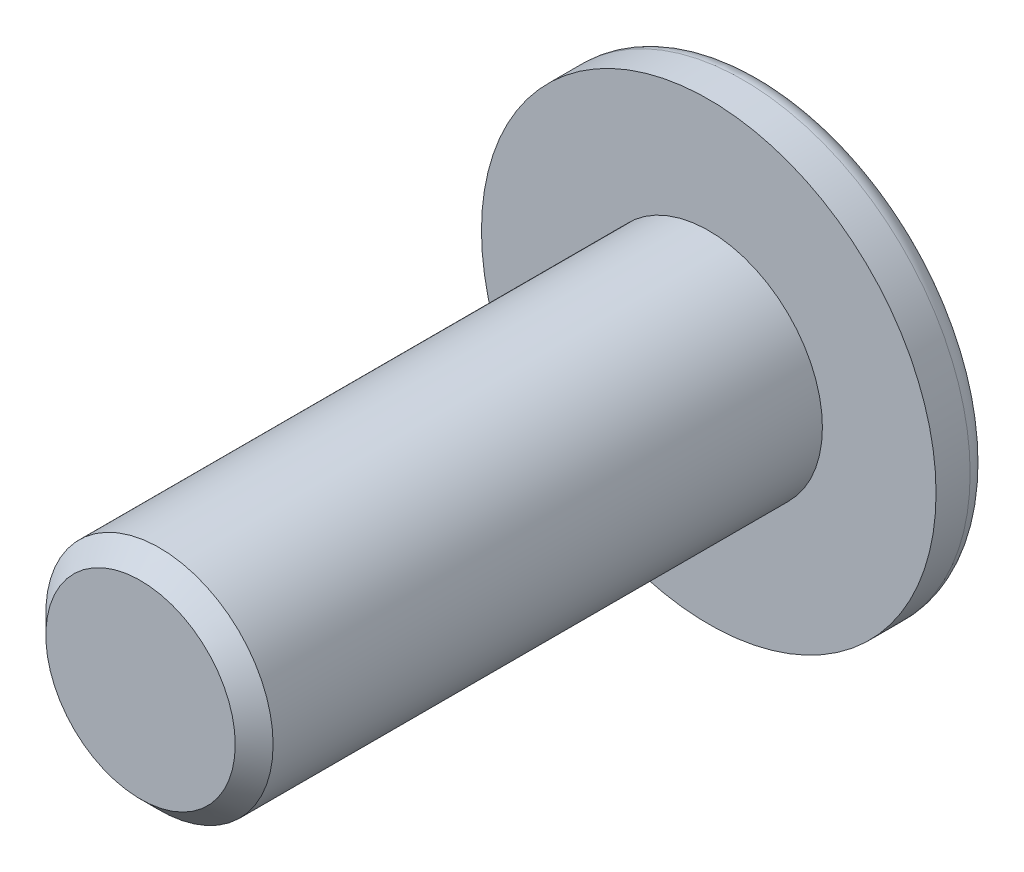
SolidWorks part; units mm, degrees
ref_plane "前视基准面" through (0, 0, 0) normal (0, 0, 1) x (1, 0, 0)
ref_plane "上视基准面" through (0, 0, 0) normal (0, 1, 0) x (1, 0, 0)
ref_plane "右视基准面" through (0, 0, 0) normal (1, 0, 0) x (0, 0, -1)
other "Configuration Table"
sketch "草图1" plane through (0, 0, 0) normal (0, 0, 1) x (1, 0, 0)
  circle A0 centre (0, 0) radius 6
  dimension "D1" = 12
extrude "凸台-拉伸1" add sketch "草图1" along normal blind 1.4
sketch "草图2" plane through (0, 0, 1.4) normal (0, 0, 1) x (1, 0, 0)
  circle A0 centre (0, 0) radius 3
  dimension "D1" = 6
extrude "凸台-拉伸2" add sketch "草图2" along normal blind 15
fillet "圆角1" radius 0.5 1 edges at (6, 0, 0)
sketch "草图3" plane through (0, 0, 0) normal (0, 0, -1) x (-1, 0, 0)
  line L1 (0.7495, -2.1844) -> (2.2665, -0.4431)
  line L2 (2.2665, -0.4431) -> (1.517, 1.7413)
  line L3 (1.517, 1.7413) -> (-0.7495, 2.1844)
  line L4 (-0.7495, 2.1844) -> (-2.2665, 0.4431)
  line L5 (-2.2665, 0.4431) -> (-1.517, -1.7413)
  line L6 (-1.517, -1.7413) -> (0.7495, -2.1844)
  circle A0 centre (0, 0) radius 2 construction
  dimension "D1" = 4
extrude "切除-拉伸1" cut sketch "草图3" against normal blind 2
chamfer "倒角1" distance 0.5 angle 45 1 edges at (3, 0, 16.4)
